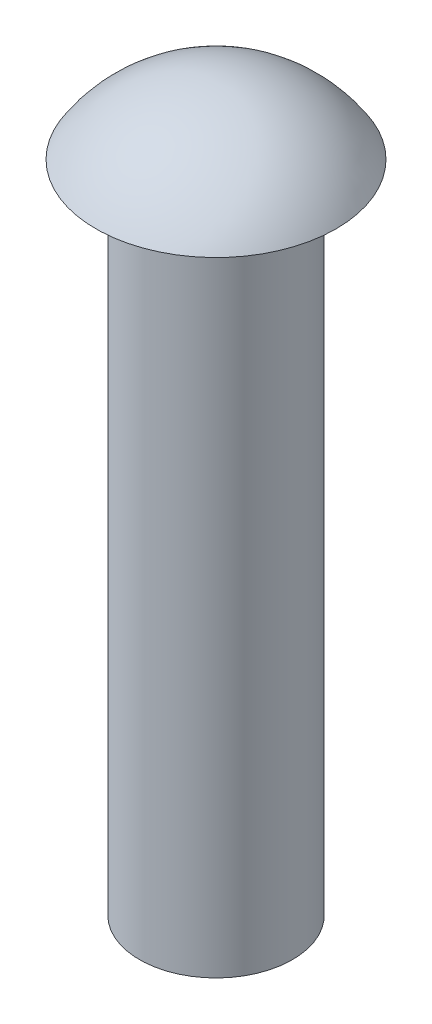
from build123d import *


with BuildPart() as part:
    # 草图1 → 旋转1 (revolve)
    with BuildSketch(Plane.XY, mode=Mode.PRIVATE) as revolve_1_sk:
        with BuildLine():
            Line((0, -15), (0, 15))
            Line((0, 15), (0, 18))
            ThreePointArc((0, 18), (3.141814541, 17.18979245), (5.5, 14.961251172))
            Line((5.5, 14.961251172), (3.5, 14.961251172))
            Line((3.5, 14.961251172), (3.5, -15))
            Line((3.5, -15), (0, -15))
        make_face()
    revolve(revolve_1_sk.sketch.rotate(Axis((0, -15, 0), (0, 1, 0)), 90), axis=Axis((0, -15, 0), (0, 1, 0)))


solid = part.part
